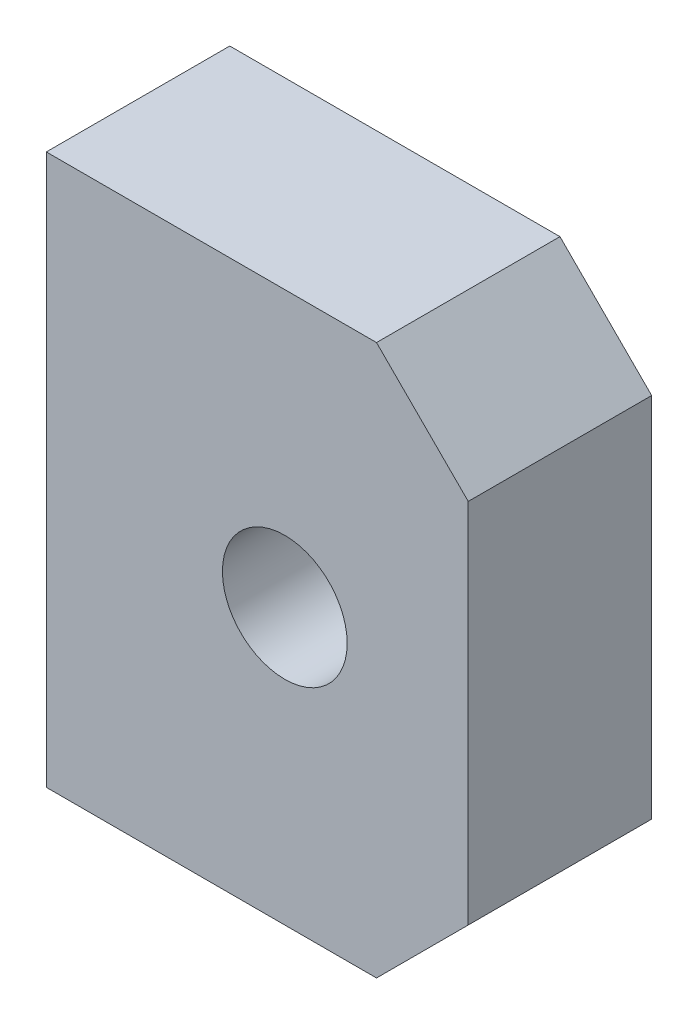
SolidWorks part; units mm, degrees
material "6061 合金"
ref_plane "前视基准面" through (0, 0, 0) normal (0, 0, 1) x (1, 0, 0)
ref_plane "上视基准面" through (0, 0, 0) normal (0, 1, 0) x (1, 0, 0)
ref_plane "右视基准面" through (0, 0, 0) normal (1, 0, 0) x (0, 0, -1)
sketch "草图1" plane through (0, 0, 0) normal (0, 0, 1) x (1, 0, 0)
  line L1 (11.5, -15) -> (-11.5, -15)
  line L2 (11.5, -15) -> (11.5, 15)
  line L3 (11.5, 15) -> (-11.5, 15)
  line L4 (-11.5, -15) -> (-11.5, 15)
  line L5 (11.5, -15) -> (-11.5, 15) construction
  line L6 (11.5, 15) -> (-11.5, -15) construction
  point P0 (0, 0)
  dimension "D1" = 23
  dimension "D2" = 30
extrude "凸台-拉伸1" add sketch "草图1" along normal blind 10
chamfer "倒角1" distance 5 angle 45 2 edges at (11.5, -15, 5) (11.5, 15, 5)
sketch "草图4" plane through (0, 0, 0) normal (0, 0, -1) x (-1, 0, 0)
  line L0 (-11.5, 0) -> (-1.5, 0) construction
  line L1 (-11.5, -10) -> (-11.5, 10) construction
  point P0 (-1.5, 0)
  dimension "D1" = 10
hole_wizard "M8 螺纹孔1" positions "草图4" profile "草图3" tap size "M8" standard "GB" end condition up to next
sketch "草图3" plane through (1.5, 0, 0) normal (1, 0, 0) x (0, 1, 0)
  line L0 (0, 0) -> (0, 10)
  line L1 (0, 10) -> (3.4, 10)
  line L2 (3.4, 10) -> (3.4, 0)
  line L5 (3.4, 0) -> (0, 0)
  line L11 (0, -6.35) -> (0, 107.95) construction
  dimension "通孔螺纹孔钻头直径" = 6.8
  dimension "通孔螺纹孔钻头深度" = 10
cosmetic thread "孔螺纹线1" parameters "D2"=8
